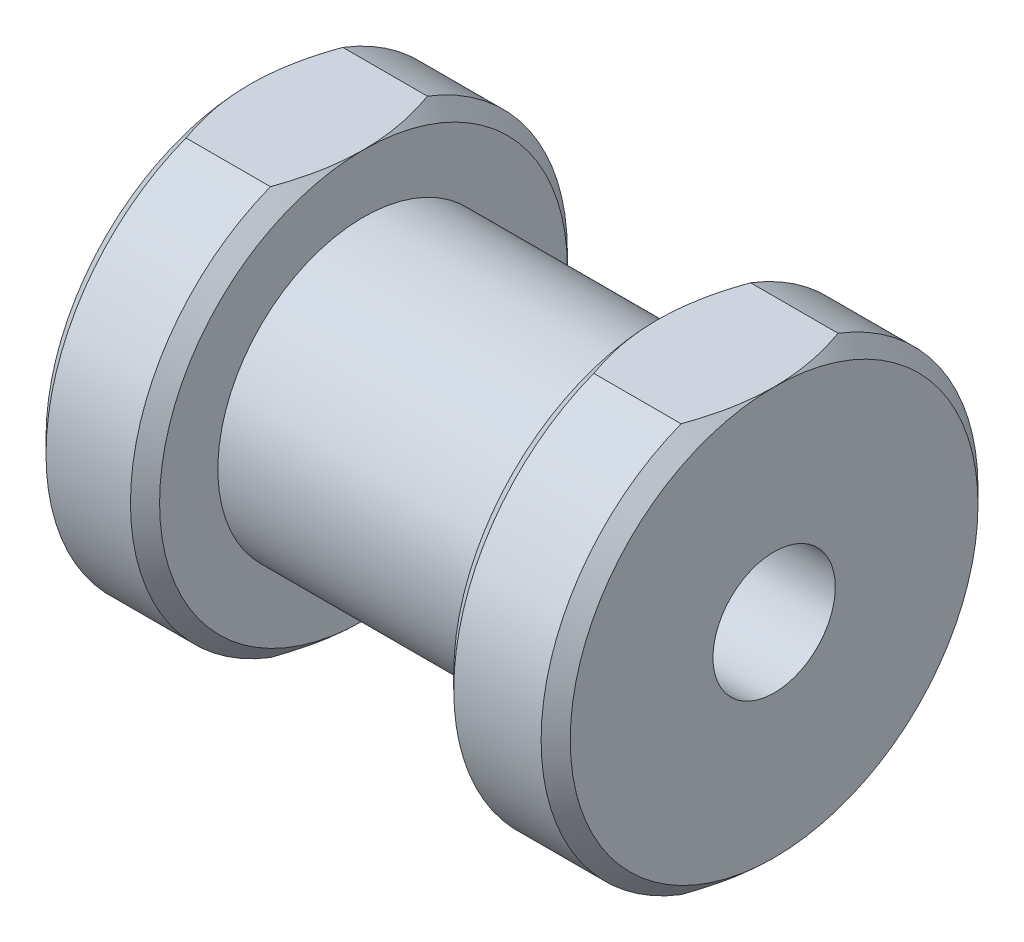
SolidWorks part; units mm, degrees
material "不锈钢"
ref_plane "Front" through (0, 0, 0) normal (0, 0, 1) x (1, 0, 0)
ref_plane "Top" through (0, 0, 0) normal (0, 1, 0) x (1, 0, 0)
ref_plane "Right" through (0, 0, 0) normal (1, 0, 0) x (0, 0, -1)
sketch "草图1" plane through (0, 0, 0) normal (1, 0, 0) x (0, 0, -1)
  circle A0 centre (0, 0) radius 7.5
  dimension "D1" = 15
extrude "凸台-拉伸1" add sketch "草图1" along normal blind 18
hole_wizard "M5 螺纹孔1" positions "草图4" profile "草图3" tap size "M5" standard "Iso" end condition through all
sketch "草图4" plane through (18, 0, 0) normal (1, 0, 0) x (0, 0, -1)
  point P0 (0, 0)
sketch "草图3" plane through (18, 0, 0) normal (0, 1, 0) x (0, 0, -1)
  line L0 (0, 0) -> (0, 18)
  line L1 (0, 18) -> (2.1, 18)
  line L2 (2.1, 18) -> (2.1, 0)
  line L5 (2.1, 0) -> (0, 0)
  line L11 (0, -6.35) -> (0, 107.95) construction
  dimension "通孔螺纹孔钻头直径" = 4.2
  dimension "通孔螺纹孔钻头深度" = 18
cosmetic thread "孔螺蚊线1" parameters "D2"=5
sketch "草图5" plane through (18, 0, 0) normal (1, 0, 0) x (0, 0, -1)
  circle A0 centre (0, 0) radius 5
  dimension "D1" = 10
extrude "切除-拉伸1" cut sketch "草图5" against normal blind 10.1 from offset 4 flip side to cut offset against normal yes
chamfer "倒角1" distance 0.5 angle 45 4 edges at (18, 0, -7.5) (14, 0, -7.5) (3.9, 0, -7.5) (0, 0, -7.5)
sketch "草图6" plane through (18, 0, 0) normal (1, 0, 0) x (0, 0, -1)
  line L1 (-15.1644, 7) -> (15.1644, 7)
  line L2 (-15.1644, 7) -> (-15.1644, -7)
  line L3 (-15.1644, -7) -> (15.1644, -7)
  line L4 (15.1644, 7) -> (15.1644, -7)
  line L5 (-15.1644, 7) -> (15.1644, -7) construction
  line L6 (-15.1644, -7) -> (15.1644, 7) construction
  point P0 (0, 0)
  dimension "D1" = 14
extrude "切除-拉伸2" cut sketch "草图6" against normal through all flip side to cut
